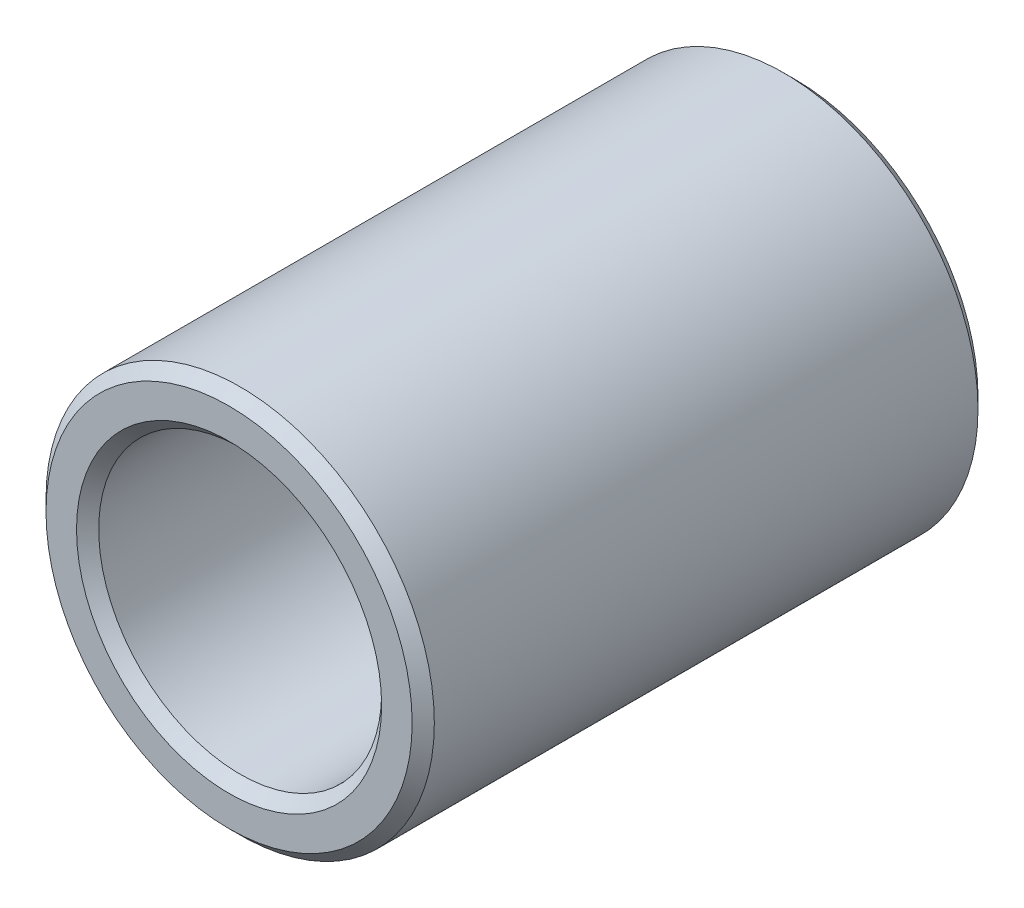
SolidWorks part; units mm, degrees
ref_plane "前视基准面" through (0, 0, 0) normal (0, 0, 1) x (1, 0, 0)
ref_plane "上视基准面" through (0, 0, 0) normal (0, 1, 0) x (1, 0, 0)
ref_plane "右视基准面" through (0, 0, 0) normal (1, 0, 0) x (0, 0, -1)
sketch "草图1" plane through (0, 0, 0) normal (0, 0, 1) x (1, 0, 0)
  circle A0 centre (0, 0) radius 12.75
  circle A1 centre (0, 0) radius 17.5
  dimension "D1" = 35
  dimension "D2" = 25.5
extrude "凸台-拉伸1" add sketch "草图1" along normal mid plane 51
chamfer "倒角1" distance 1 angle 45 4 edges at (17.5, 0, -25.5) (12.75, 0, -25.5) (12.75, 0, 25.5) (17.5, 0, 25.5)
